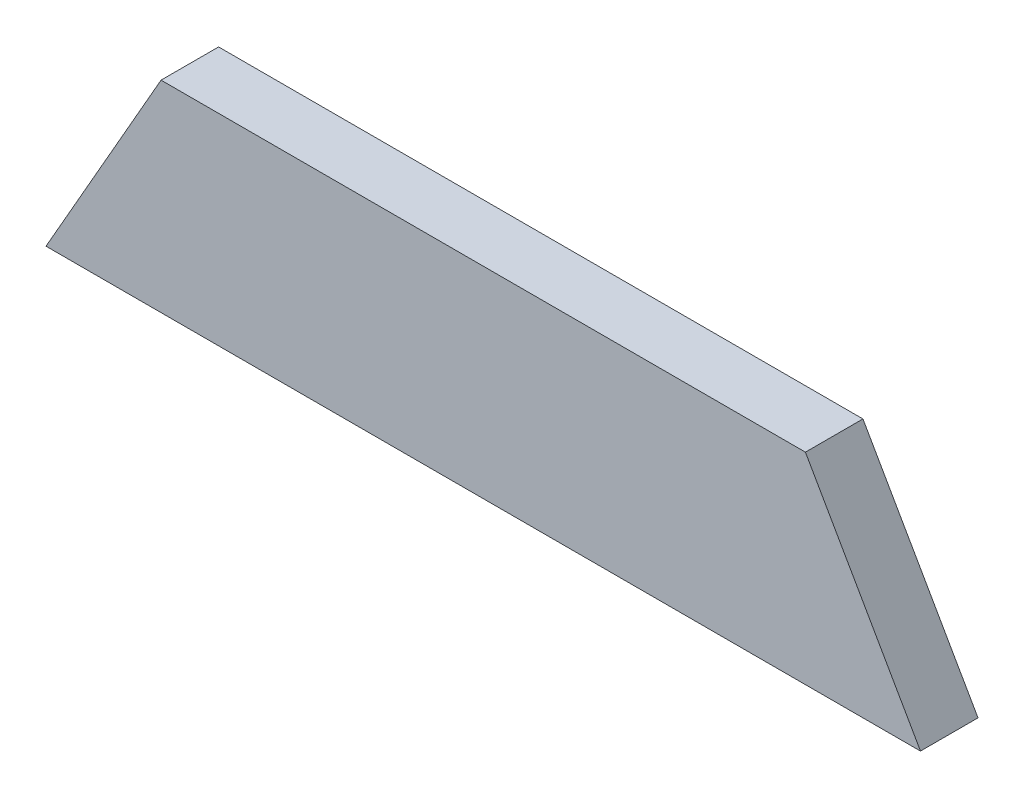
SolidWorks part; units mm, degrees
ref_plane "Front Plane" through (0, 0, 0) normal (0, 0, 1) x (1, 0, 0)
ref_plane "Top Plane" through (0, 0, 0) normal (0, 1, 0) x (1, 0, 0)
ref_plane "Right Plane" through (0, 0, 0) normal (1, 0, 0) x (0, 0, -1)
other "Configuration Table"
sketch "Sketch1" plane through (0, 0, 0) normal (0, 0, 1) x (1, 0, 0)
  line L0 (0, 0) -> (152, 0)
  line L1 (152, 0) -> (132, 35)
  line L2 (132, 35) -> (20, 35)
  line L3 (20, 35) -> (0, 0)
  line L4 (76, 0) -> (76, 35) construction
  dimension "D1" = 112
  dimension "D2" = 152
  dimension "D3" = 35
extrude "Boss-Extrude1" add sketch "Sketch1" along normal blind 10
